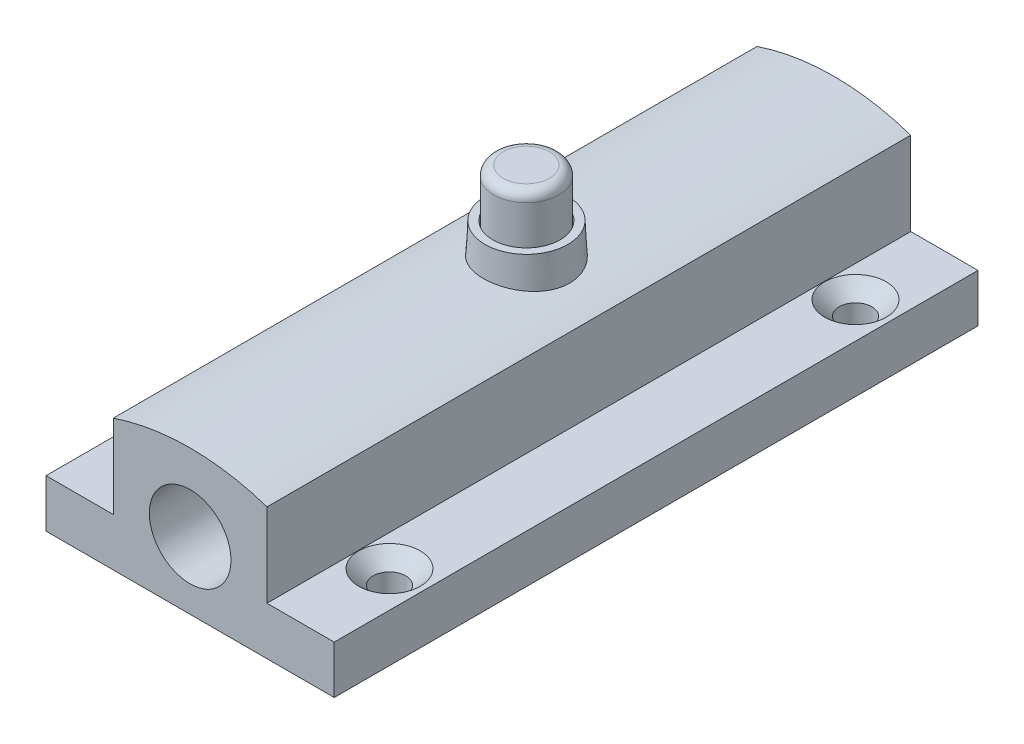
SolidWorks part; units mm, degrees
material "AL6061"
ref_plane "前视基准面" through (0, 0, 0) normal (0, 0, 1) x (1, 0, 0)
ref_plane "上视基准面" through (0, 0, 0) normal (0, 1, 0) x (1, 0, 0)
ref_plane "右视基准面" through (0, 0, 0) normal (1, 0, 0) x (0, 0, -1)
sketch "草图1" plane through (0, 0, 0) normal (0, 0, 1) x (1, 0, 0)
  line L0 (-18.0481, 0) -> (16.7647, 0) construction
  line L1 (0, 9.4652) -> (0, -8.3422) construction
  line L2 (-15, 5) -> (-8, 5)
  line L3 (8, 5) -> (8, 13.6854)
  line L4 (-15, 5) -> (-15, 0)
  line L5 (-15, 0) -> (15, 0)
  line L6 (15, 5) -> (15, 0)
  line L7 (-8, 5) -> (-8, 13.6854)
  line L8 (15, 5) -> (8, 5)
  arc A0 (-8, 13.6854) -> (8, 13.6854) centre (0, -10) cw
  dimension "D4" = 15
  dimension "D5" = 25
  dimension "D1" = 30
  dimension "D2" = 5
  dimension "D3" = 16
extrude "凸台-拉伸1" add sketch "草图1" along normal mid plane 67
hole_wizard "打孔尺寸开槽半沉头螺钉的类型1" positions "草图2" profile "草图3" countersink size "M3" standard "GB" end condition through all
sketch "草图2" plane through (0, 5, 0) normal (0, 1, 0) x (1, 0, 0)
  line L0 (0, 32.3351) -> (0, -35.9769) construction
  line L1 (-8, 33.5) -> (-15, 33.5) construction
  point P0 (-11.25, 24.5)
  point P2 (-11.25, -24)
  point P9 (11.25, -24)
  point P10 (11.25, 24.5)
  dimension "D1" = 48.5
  dimension "D2" = 22.5
  dimension "D3" = 9
sketch "草图3" plane through (-11.25, 5, -24.5) normal (1, 0, 0) x (0, 0, 1)
  line L0 (0, 0) -> (0, 5)
  line L1 (0, 5) -> (1.7, 5)
  line L2 (1.7, 5) -> (1.7, 1.5)
  line L3 (1.7, 1.5) -> (3.2, 0)
  line L5 (3.2, 0) -> (0, 0)
  line L6 (-1.7, 1.5) -> (-3.2, 0) construction
  line L11 (0, -6.35) -> (0, 107.95) construction
  dimension "通孔孔直径" = 3.4
  dimension "通孔孔深度" = 5
  dimension "近端锥形沉头孔直径" = 6.4
  dimension "近端锥形沉头孔角度" = 90
sketch "草图4" plane through (0, 5, 0) normal (0, 1, 0) x (1, 0, 0)
  line L0 (0, 35.24) -> (0, -37.9603) construction
  line L1 (15, 33.5) -> (8, 33.5) construction
  circle A0 centre (0, 1.5) radius 5
  dimension "D1" = 32
  dimension "D2" = 10
extrude "凸台-拉伸2" add sketch "草图4" along normal blind 13 draft 3
sketch "草图6" plane through (0, 18, 0) normal (0, 1, 0) x (1, 0, 0)
  circle A0 centre (0, 1.5) radius 3.5
  dimension "D1" = 7
extrude "切除-拉伸2" cut sketch "草图6" against normal blind 7
sketch "草图5" plane through (0, 0, 33.5) normal (0, 0, 1) x (1, 0, 0)
  line L0 (0, 14.8719) -> (0, -1.5564) construction
  line L1 (-15, 0) -> (15, 0) construction
  circle A0 centre (0, 7) radius 4.25
  dimension "D1" = 7
  dimension "D2" = 8.5
extrude "切除-拉伸1" cut sketch "草图5" against normal through all
sketch "草图7" plane through (0, 18, 0) normal (0, 1, 0) x (1, 0, 0)
  circle A0 centre (0, 1.5) radius 3.4
  dimension "D1" = 6.8
extrude "凸台-拉伸3" add sketch "草图7" along normal mid plane 10 separate body
fillet "圆角1" radius 1 1 edges at (0, 23, 1.9)
